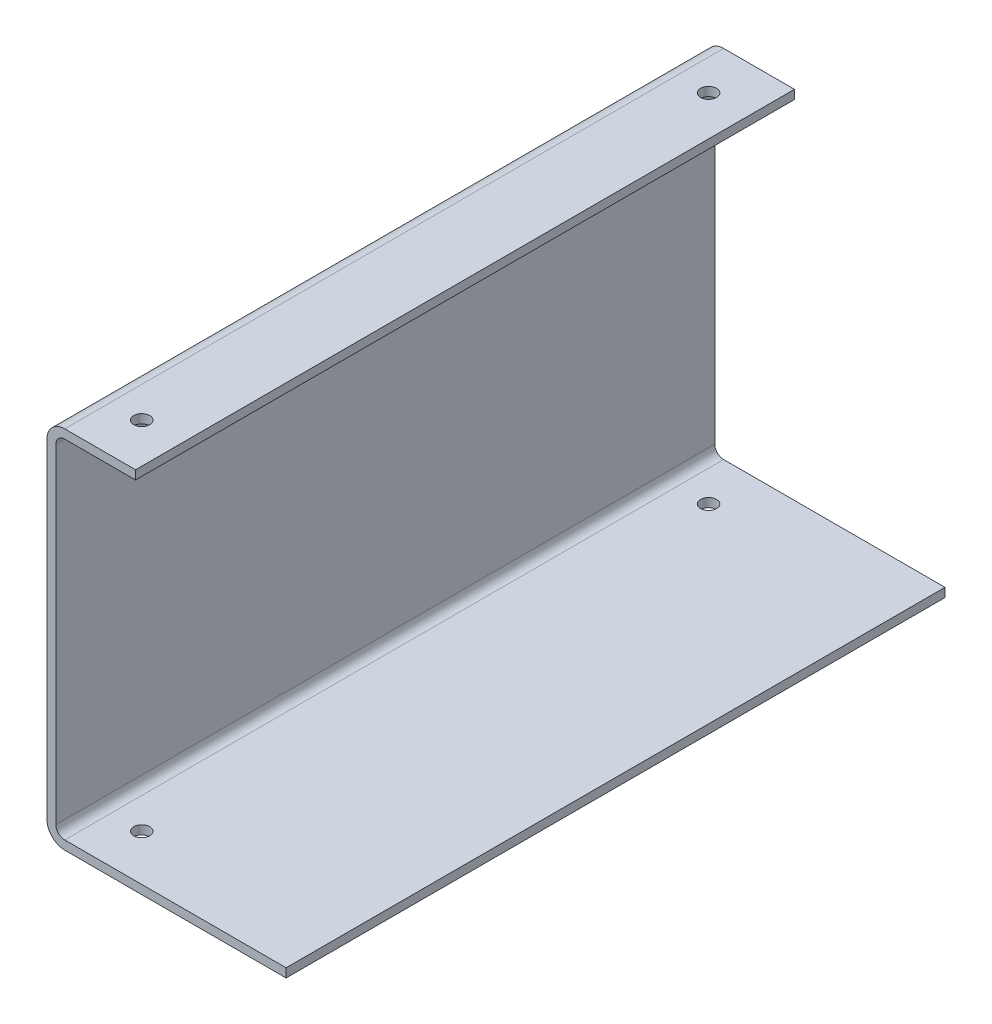
SolidWorks part; units mm, degrees
material "Plain Carbon Steel"
ref_plane "Front Plane" through (0, 0, 0) normal (0, 0, 1) x (1, 0, 0)
ref_plane "Top Plane" through (0, 0, 0) normal (0, 1, 0) x (1, 0, 0)
ref_plane "Right Plane" through (0, 0, 0) normal (1, 0, 0) x (0, 0, -1)
sketch "Sketch1" plane through (0, 0, 0) normal (0, 0, 1) x (1, 0, 0)
  line L0 (10, 0) -> (135, 0)
  line L1 (0, 10) -> (0, 196)
  line L2 (10, 206) -> (50, 206)
  arc A0 (10, 0) -> (0, 10) centre (10, 10) cw
  arc A1 (10, 206) -> (0, 196) centre (10, 196) ccw
  point P7 (0, 0)
  point P10 (0, 206)
  dimension "D4" = 10
  dimension "D1" = 206
  dimension "D2" = 50
  dimension "D3" = 135
extrude "Extrude-Thin1" add sketch "Sketch1" along normal blind 372 thin thin type one direction wall 5
sketch "Sketch2" plane through (0, 206, 0) normal (0, 1, 0) x (1, 0, 0)
  line L0 (0, -372) -> (0, 0) construction
  line L1 (10, -372) -> (50, -372) construction
  circle A0 centre (27.5, -346) radius 4.5
  dimension "D3" = 9
  dimension "D1" = 27.5
  dimension "D2" = 26
extrude "Cut-Extrude1" cut sketch "Sketch2" against normal through all
pattern_linear "LPattern1" count 2 spacing 320 along (0, 0, -1) of "Cut-Extrude1"
